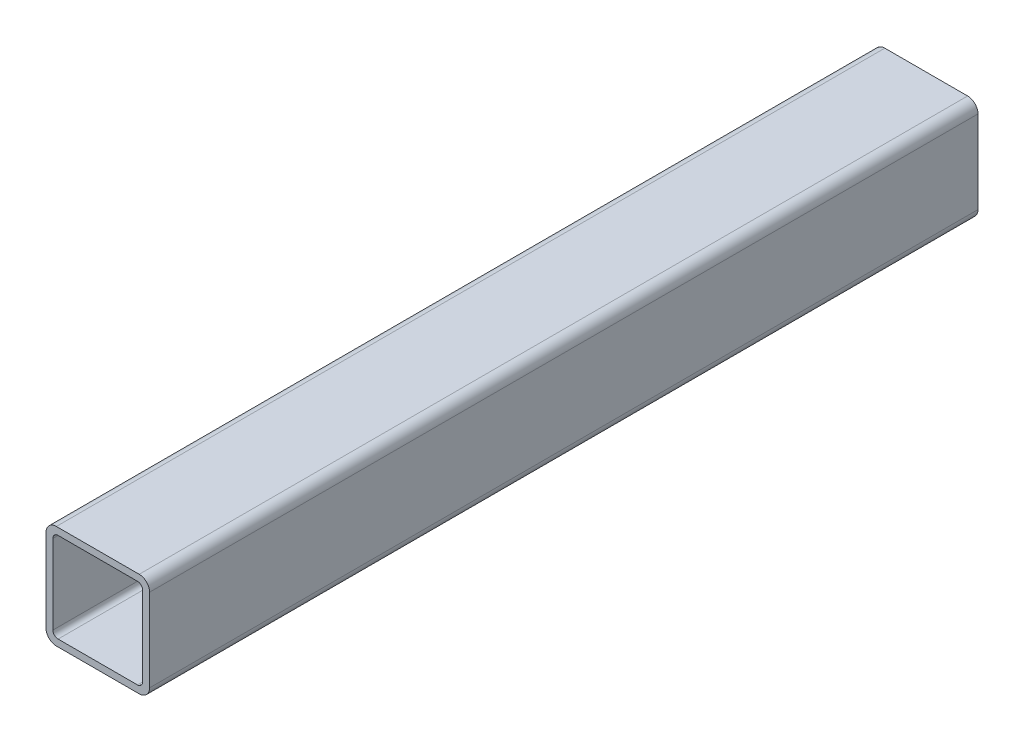
SolidWorks part; units mm, degrees
material "Q235"
ref_plane "Front Plane" through (0, 0, 0) normal (0, 0, 1) x (1, 0, 0)
ref_plane "Top Plane" through (0, 0, 0) normal (0, 1, 0) x (1, 0, 0)
ref_plane "Right Plane" through (0, 0, 0) normal (1, 0, 0) x (0, 0, -1)
sketch "Sketch1" plane through (0, 0, 0) normal (0, 0, 1) x (1, 0, 0)
  line L1 (-30, -30) -> (30, -30)
  line L2 (-30, -30) -> (-30, 30)
  line L3 (-30, 30) -> (30, 30)
  line L4 (30, -30) -> (30, 30)
  line L5 (-30, -30) -> (30, 30) construction
  line L6 (-30, 30) -> (30, -30) construction
  line L7 (-26, -26) -> (26, -26)
  line L8 (-26, -26) -> (-26, 26)
  line L9 (-26, 26) -> (26, 26)
  line L10 (26, -26) -> (26, 26)
  line L11 (-26, -26) -> (26, 26) construction
  line L12 (-26, 26) -> (26, -26) construction
  point P0 (0, 0)
  point P5 (0, 0)
  dimension "D1" = 4
  dimension "D2" = 60
  dimension "D3" = 60
extrude "Boss-Extrude1" add sketch "Sketch1" along normal mid plane 480
fillet "Fillet1" radius 6 4 edges at (30, -30, 0) (-30, -30, 0) (30, 30, 0) (-30, 30, 0)
fillet "Fillet2" radius 3 4 edges at (26, -26, 0) (-26, -26, 0) (26, 26, 0) (-26, 26, 0)
